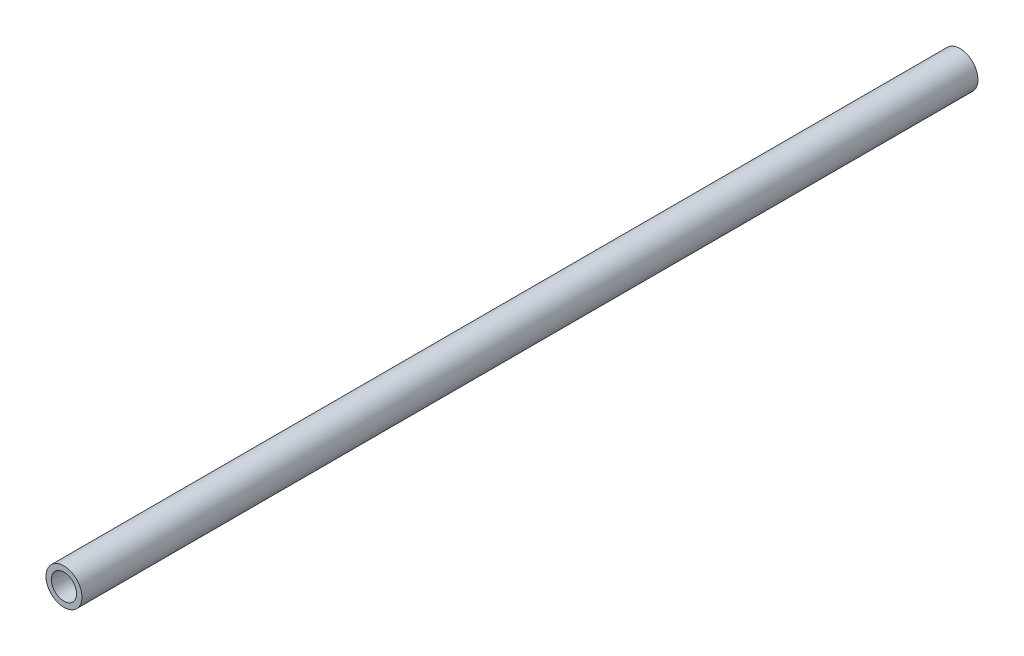
from build123d import *

# Parameters (mm, degrees)
BOSS_EXTRUDE1_DEPTH      = 462
BOSS_EXTRUDE1_DEPTH_BACK = 36
SKETCH4_R                = 10
SKETCH5_R                = 7
CUT_EXTRUDE1_DEPTH       = 500.105615354


with BuildPart() as part:
    # Sketch4 → Boss-Extrude1 (new, two sides: drawn at the far end of the back side and taken through both)
    with BuildSketch(Plane.XY.offset(-BOSS_EXTRUDE1_DEPTH_BACK)):
        with Locations((16.5, -10.004131531)):
            Circle(SKETCH4_R)
    extrude(amount=BOSS_EXTRUDE1_DEPTH + BOSS_EXTRUDE1_DEPTH_BACK)

    # Sketch5 → Cut-Extrude1 (cut, through all)
    with BuildSketch(Plane(origin=(0, 0, -36), x_dir=(-1, 0, 0), z_dir=(0, 0, -1))):
        with Locations((-16.5, -10.004131531)):
            Circle(SKETCH5_R)
    extrude(amount=-CUT_EXTRUDE1_DEPTH, mode=Mode.SUBTRACT)


solid = part.part
